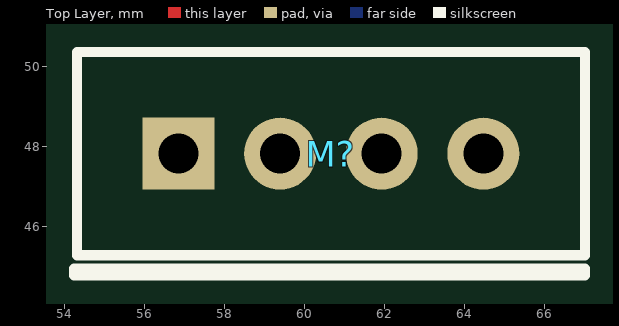
[diagram p0: Top Layer view]
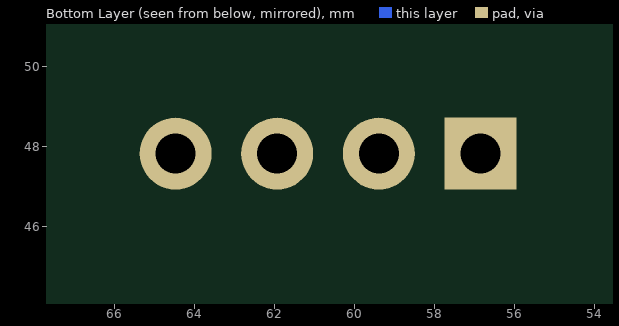
[diagram p1: Bottom Layer view, seen from below]
# Altium PCB MISC84237-7.PcbDoc
Units mm, origin at the board's own origin, x right, y up, seen from the top; angles counter-clockwise.
Board outline 71.29 x 45.91 mm, 2 copper layers (Top Layer, Bottom Layer); 1 components, 0 nets, 4 pads, 0 vias.

## Layer stack, top to bottom (the 12.6 mil dielectric is the usual default, probably not edited)
Top Layer: signal copper (thickness not stored)
Dielectric: dielectric 0.32, FR-4, Dk 4.8
Bottom Layer: signal copper (thickness not stored)

## Board outline
96.689,25.4 25.4,25.4 25.4,71.312 96.689,71.312

## Components (designator, comment, footprint, x,y, rotation, side; value= is the part's Value field where it differs from the comment)
M? "HC-SR04" HC-SR04 60.6,48.229 r0 top

## Footprints (in the part's own frame and the unit in brackets; to place one, negate y for a bottom-side part, rotate by r counter-clockwise, add the part's x,y. Pads: shape width x height; smd on the part's side, far side on the other; paste and mask are expansions set on the pad)
HC-SR04 [mm]
  rect 1.8x1.8 hole 1 paste+0 mask+0.102: 1(-3.742,-0.411)
  round 1.8 hole 1 paste+0 mask+0.102: 2(-1.202,-0.411) 3(1.338,-0.411) 4(3.878,-0.411)
  silkscreen extent -6.36,-3.46 6.42,2.13

## Nets (pads, with @x,y where several pads share a name; then routed paths per layer and width w, separated by ;. In a path a pad name is that pad's centre, name@x,y a point inside that pad or via, vN(x,y) a via of type N, cw(c..) or ccw(c..) an arc to the next point about the centre after c; other vN are vias at no path point)
pads on no net: M?.1 M?.2 M?.3 M?.4

## Silkscreen, mask and mechanical layers (free items; w line width, h text height)
Document:
  lines w0.003: 61.044,48.356 61.045,48.356